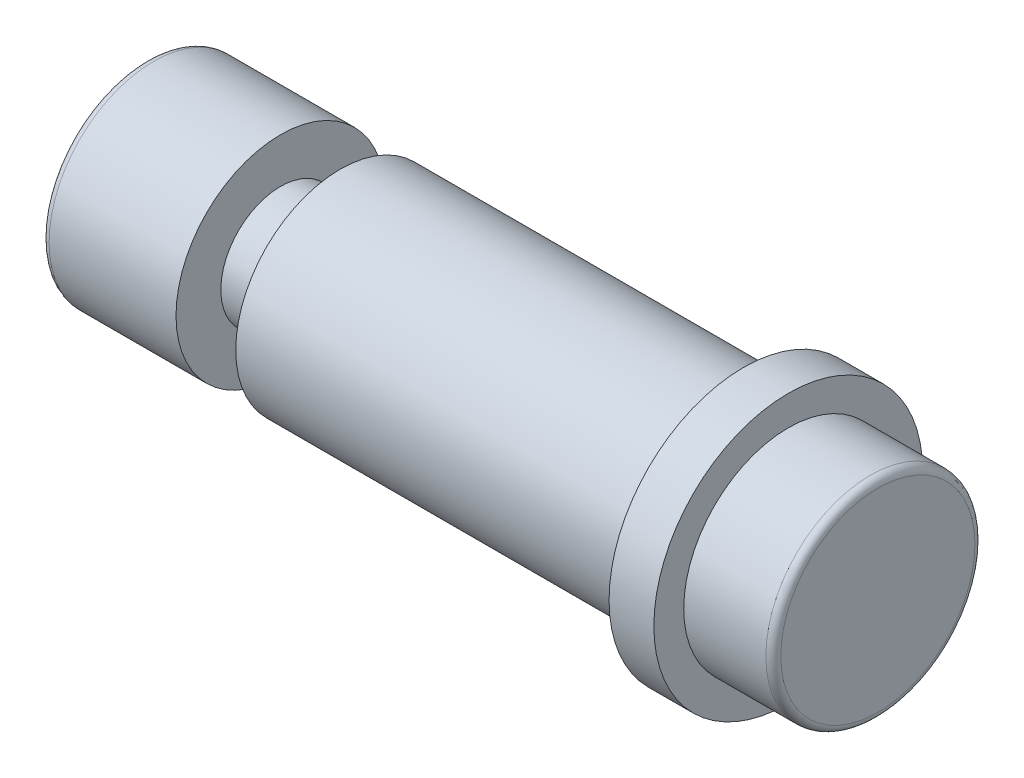
SolidWorks part; units mm, degrees
ref_plane "Front Plane" through (0, 0, 0) normal (0, 0, 1) x (1, 0, 0)
ref_plane "Top Plane" through (0, 0, 0) normal (0, 1, 0) x (1, 0, 0)
ref_plane "Right Plane" through (0, 0, 0) normal (1, 0, 0) x (0, 0, -1)
sketch "Sketch1" plane through (0, 0, 0) normal (0, 0, 1) x (1, 0, 0)
  line L0 (0, 0) -> (0, 7)
  line L1 (0, 7) -> (9, 7)
  line L2 (9, 7) -> (9, 4)
  line L3 (9, 4) -> (13, 4)
  line L4 (13, 4) -> (13, 7)
  line L5 (13, 7) -> (40, 7)
  line L6 (40, 7) -> (40, 9)
  line L7 (40, 9) -> (43, 9)
  line L8 (43, 9) -> (43, 7)
  line L9 (43, 7) -> (49, 7)
  line L10 (49, 7) -> (49, 0)
  line L11 (49, 0) -> (0, 0)
  dimension "D1" = 49
  dimension "D2" = 4
  dimension "D3" = 7
  dimension "D4" = 4
  dimension "D5" = 27
  dimension "D6" = 3
  dimension "D7" = 6
  dimension "D8" = 9
  dimension "D9" = 7
revolve "Revolve1" add sketch "Sketch1" angle 360 about L11
fillet "Fillet1" radius 0.5 2 edges at (0, 0, -7) (49, 0, -7)
